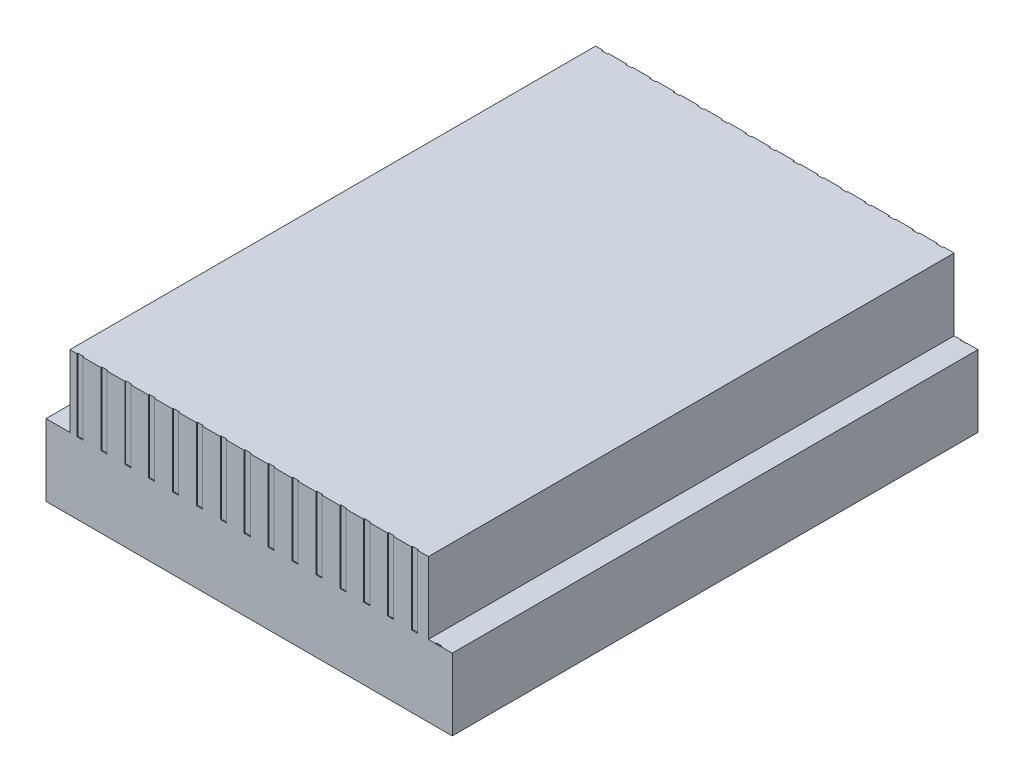
from build123d import *

# Parameters (mm, degrees)
BOSS_EXTRUDE1_DEPTH      = 110
SKETCH2_W                = 1.259860676
SKETCH2_H                = 15.043092937
CUT_EXTRUDE1_DEPTH       = 0.2
LPATTERN1_COUNT          = 16
LPATTERN1_PITCH          = 5
MIRROR1_COPY_1_SKETCH_W  = 1.259860676
MIRROR1_COPY_1_SKETCH_H  = 15.043092937
MIRROR1_COPY_1_DEPTH     = 0.2
MIRROR1_COPY_2_SKETCH_W  = 1.259860676
MIRROR1_COPY_2_SKETCH_H  = 15.043092937
MIRROR1_COPY_2_DEPTH     = 0.2
MIRROR1_COPY_3_SKETCH_W  = 1.259860676
MIRROR1_COPY_3_SKETCH_H  = 15.043092937
MIRROR1_COPY_3_DEPTH     = 0.2
MIRROR1_COPY_4_SKETCH_W  = 1.259860676
MIRROR1_COPY_4_SKETCH_H  = 15.043092937
MIRROR1_COPY_4_DEPTH     = 0.2
MIRROR1_COPY_5_SKETCH_W  = 1.259860676
MIRROR1_COPY_5_SKETCH_H  = 15.043092937
MIRROR1_COPY_5_DEPTH     = 0.2
MIRROR1_COPY_6_SKETCH_W  = 1.259860676
MIRROR1_COPY_6_SKETCH_H  = 15.043092937
MIRROR1_COPY_6_DEPTH     = 0.2
MIRROR1_COPY_7_SKETCH_W  = 1.259860676
MIRROR1_COPY_7_SKETCH_H  = 15.043092937
MIRROR1_COPY_7_DEPTH     = 0.2
MIRROR1_COPY_8_SKETCH_W  = 1.259860676
MIRROR1_COPY_8_SKETCH_H  = 15.043092937
MIRROR1_COPY_8_DEPTH     = 0.2
MIRROR1_COPY_9_SKETCH_W  = 1.259860676
MIRROR1_COPY_9_SKETCH_H  = 15.043092937
MIRROR1_COPY_9_DEPTH     = 0.2
MIRROR1_COPY_10_SKETCH_W = 1.259860676
MIRROR1_COPY_10_SKETCH_H = 15.043092937
MIRROR1_COPY_10_DEPTH    = 0.2
MIRROR1_COPY_11_SKETCH_W = 1.259860676
MIRROR1_COPY_11_SKETCH_H = 15.043092937
MIRROR1_COPY_11_DEPTH    = 0.2
MIRROR1_COPY_12_SKETCH_W = 1.259860676
MIRROR1_COPY_12_SKETCH_H = 15.043092937
MIRROR1_COPY_12_DEPTH    = 0.2
MIRROR1_COPY_13_SKETCH_W = 1.259860676
MIRROR1_COPY_13_SKETCH_H = 15.043092937
MIRROR1_COPY_13_DEPTH    = 0.2
MIRROR1_COPY_14_SKETCH_W = 1.259860676
MIRROR1_COPY_14_SKETCH_H = 15.043092937
MIRROR1_COPY_14_DEPTH    = 0.2
MIRROR1_COPY_15_SKETCH_W = 1.259860676
MIRROR1_COPY_15_SKETCH_H = 15.043092937
MIRROR1_COPY_15_DEPTH    = 0.2
SKETCH4_W                = 38.958676741
SKETCH4_H                = 137.401414086
CUT_EXTRUDE2_DEPTH       = 192.049731745


with BuildPart() as part:
    # Sketch1 → Boss-Extrude1 (new body)
    with BuildSketch(Plane.XY):
        Polygon((0, 0), (100, 0), (100, 15), (95, 15), (95, 30), (20, 30), (20, 15), (15, 15), (15, 120), (0, 120), align=None)
    extrude(amount=BOSS_EXTRUDE1_DEPTH)

    # Sketch2 → Cut-Extrude1 (cut)
    with BuildSketch(Plane.XY.offset(110)):
        with Locations((22.109179897, 22.478453532)):
            Rectangle(SKETCH2_W, SKETCH2_H)
    cut_extrude1 = extrude(amount=-CUT_EXTRUDE1_DEPTH, mode=Mode.SUBTRACT)

    # LPattern1: Cut-Extrude1 ×16
    with Locations(*[(i * LPATTERN1_PITCH, 0, 0) for i in range(1, LPATTERN1_COUNT)]):
        add(cut_extrude1, mode=Mode.SUBTRACT)

    # Mirror1: Cut-Extrude1 across plane
    add(cut_extrude1.mirror(Plane(origin=(0, 0, 55), x_dir=(1, 0, 0), z_dir=(0, 0, -1))), mode=Mode.SUBTRACT)

    # Mirror1 copy 1 sketch → Mirror1 copy 1 (cut)
    with BuildSketch(Plane(origin=(5, 0, 0), x_dir=(1, 0, 0), z_dir=(0, 0, -1))):
        with Locations((22.109179897, -22.478453532)):
            Rectangle(MIRROR1_COPY_1_SKETCH_W, MIRROR1_COPY_1_SKETCH_H)
    extrude(amount=-MIRROR1_COPY_1_DEPTH, mode=Mode.SUBTRACT)

    # Mirror1 copy 2 sketch → Mirror1 copy 2 (cut)
    with BuildSketch(Plane(origin=(10, 0, 0), x_dir=(1, 0, 0), z_dir=(0, 0, -1))):
        with Locations((22.109179897, -22.478453532)):
            Rectangle(MIRROR1_COPY_2_SKETCH_W, MIRROR1_COPY_2_SKETCH_H)
    extrude(amount=-MIRROR1_COPY_2_DEPTH, mode=Mode.SUBTRACT)

    # Mirror1 copy 3 sketch → Mirror1 copy 3 (cut)
    with BuildSketch(Plane(origin=(15, 0, 0), x_dir=(1, 0, 0), z_dir=(0, 0, -1))):
        with Locations((22.109179897, -22.478453532)):
            Rectangle(MIRROR1_COPY_3_SKETCH_W, MIRROR1_COPY_3_SKETCH_H)
    extrude(amount=-MIRROR1_COPY_3_DEPTH, mode=Mode.SUBTRACT)

    # Mirror1 copy 4 sketch → Mirror1 copy 4 (cut)
    with BuildSketch(Plane(origin=(20, 0, 0), x_dir=(1, 0, 0), z_dir=(0, 0, -1))):
        with Locations((22.109179897, -22.478453532)):
            Rectangle(MIRROR1_COPY_4_SKETCH_W, MIRROR1_COPY_4_SKETCH_H)
    extrude(amount=-MIRROR1_COPY_4_DEPTH, mode=Mode.SUBTRACT)

    # Mirror1 copy 5 sketch → Mirror1 copy 5 (cut)
    with BuildSketch(Plane(origin=(25, 0, 0), x_dir=(1, 0, 0), z_dir=(0, 0, -1))):
        with Locations((22.109179897, -22.478453532)):
            Rectangle(MIRROR1_COPY_5_SKETCH_W, MIRROR1_COPY_5_SKETCH_H)
    extrude(amount=-MIRROR1_COPY_5_DEPTH, mode=Mode.SUBTRACT)

    # Mirror1 copy 6 sketch → Mirror1 copy 6 (cut)
    with BuildSketch(Plane(origin=(30, 0, 0), x_dir=(1, 0, 0), z_dir=(0, 0, -1))):
        with Locations((22.109179897, -22.478453532)):
            Rectangle(MIRROR1_COPY_6_SKETCH_W, MIRROR1_COPY_6_SKETCH_H)
    extrude(amount=-MIRROR1_COPY_6_DEPTH, mode=Mode.SUBTRACT)

    # Mirror1 copy 7 sketch → Mirror1 copy 7 (cut)
    with BuildSketch(Plane(origin=(35, 0, 0), x_dir=(1, 0, 0), z_dir=(0, 0, -1))):
        with Locations((22.109179897, -22.478453532)):
            Rectangle(MIRROR1_COPY_7_SKETCH_W, MIRROR1_COPY_7_SKETCH_H)
    extrude(amount=-MIRROR1_COPY_7_DEPTH, mode=Mode.SUBTRACT)

    # Mirror1 copy 8 sketch → Mirror1 copy 8 (cut)
    with BuildSketch(Plane(origin=(40, 0, 0), x_dir=(1, 0, 0), z_dir=(0, 0, -1))):
        with Locations((22.109179897, -22.478453532)):
            Rectangle(MIRROR1_COPY_8_SKETCH_W, MIRROR1_COPY_8_SKETCH_H)
    extrude(amount=-MIRROR1_COPY_8_DEPTH, mode=Mode.SUBTRACT)

    # Mirror1 copy 9 sketch → Mirror1 copy 9 (cut)
    with BuildSketch(Plane(origin=(45, 0, 0), x_dir=(1, 0, 0), z_dir=(0, 0, -1))):
        with Locations((22.109179897, -22.478453532)):
            Rectangle(MIRROR1_COPY_9_SKETCH_W, MIRROR1_COPY_9_SKETCH_H)
    extrude(amount=-MIRROR1_COPY_9_DEPTH, mode=Mode.SUBTRACT)

    # Mirror1 copy 10 sketch → Mirror1 copy 10 (cut)
    with BuildSketch(Plane(origin=(50, 0, 0), x_dir=(1, 0, 0), z_dir=(0, 0, -1))):
        with Locations((22.109179897, -22.478453532)):
            Rectangle(MIRROR1_COPY_10_SKETCH_W, MIRROR1_COPY_10_SKETCH_H)
    extrude(amount=-MIRROR1_COPY_10_DEPTH, mode=Mode.SUBTRACT)

    # Mirror1 copy 11 sketch → Mirror1 copy 11 (cut)
    with BuildSketch(Plane(origin=(55, 0, 0), x_dir=(1, 0, 0), z_dir=(0, 0, -1))):
        with Locations((22.109179897, -22.478453532)):
            Rectangle(MIRROR1_COPY_11_SKETCH_W, MIRROR1_COPY_11_SKETCH_H)
    extrude(amount=-MIRROR1_COPY_11_DEPTH, mode=Mode.SUBTRACT)

    # Mirror1 copy 12 sketch → Mirror1 copy 12 (cut)
    with BuildSketch(Plane(origin=(60, 0, 0), x_dir=(1, 0, 0), z_dir=(0, 0, -1))):
        with Locations((22.109179897, -22.478453532)):
            Rectangle(MIRROR1_COPY_12_SKETCH_W, MIRROR1_COPY_12_SKETCH_H)
    extrude(amount=-MIRROR1_COPY_12_DEPTH, mode=Mode.SUBTRACT)

    # Mirror1 copy 13 sketch → Mirror1 copy 13 (cut)
    with BuildSketch(Plane(origin=(65, 0, 0), x_dir=(1, 0, 0), z_dir=(0, 0, -1))):
        with Locations((22.109179897, -22.478453532)):
            Rectangle(MIRROR1_COPY_13_SKETCH_W, MIRROR1_COPY_13_SKETCH_H)
    extrude(amount=-MIRROR1_COPY_13_DEPTH, mode=Mode.SUBTRACT)

    # Mirror1 copy 14 sketch → Mirror1 copy 14 (cut)
    with BuildSketch(Plane(origin=(70, 0, 0), x_dir=(1, 0, 0), z_dir=(0, 0, -1))):
        with Locations((22.109179897, -22.478453532)):
            Rectangle(MIRROR1_COPY_14_SKETCH_W, MIRROR1_COPY_14_SKETCH_H)
    extrude(amount=-MIRROR1_COPY_14_DEPTH, mode=Mode.SUBTRACT)

    # Mirror1 copy 15 sketch → Mirror1 copy 15 (cut)
    with BuildSketch(Plane(origin=(75, 0, 0), x_dir=(1, 0, 0), z_dir=(0, 0, -1))):
        with Locations((22.109179897, -22.478453532)):
            Rectangle(MIRROR1_COPY_15_SKETCH_W, MIRROR1_COPY_15_SKETCH_H)
    extrude(amount=-MIRROR1_COPY_15_DEPTH, mode=Mode.SUBTRACT)

    # Sketch4 → Cut-Extrude2 (cut, through all)
    with BuildSketch(Plane(origin=(0, 0, 0), x_dir=(-1, 0, 0), z_dir=(0, 0, -1))):
        with Locations((4.47933837, 51.299292957)):
            Rectangle(SKETCH4_W, SKETCH4_H)
    extrude(amount=-CUT_EXTRUDE2_DEPTH, mode=Mode.SUBTRACT)


solid = part.part
